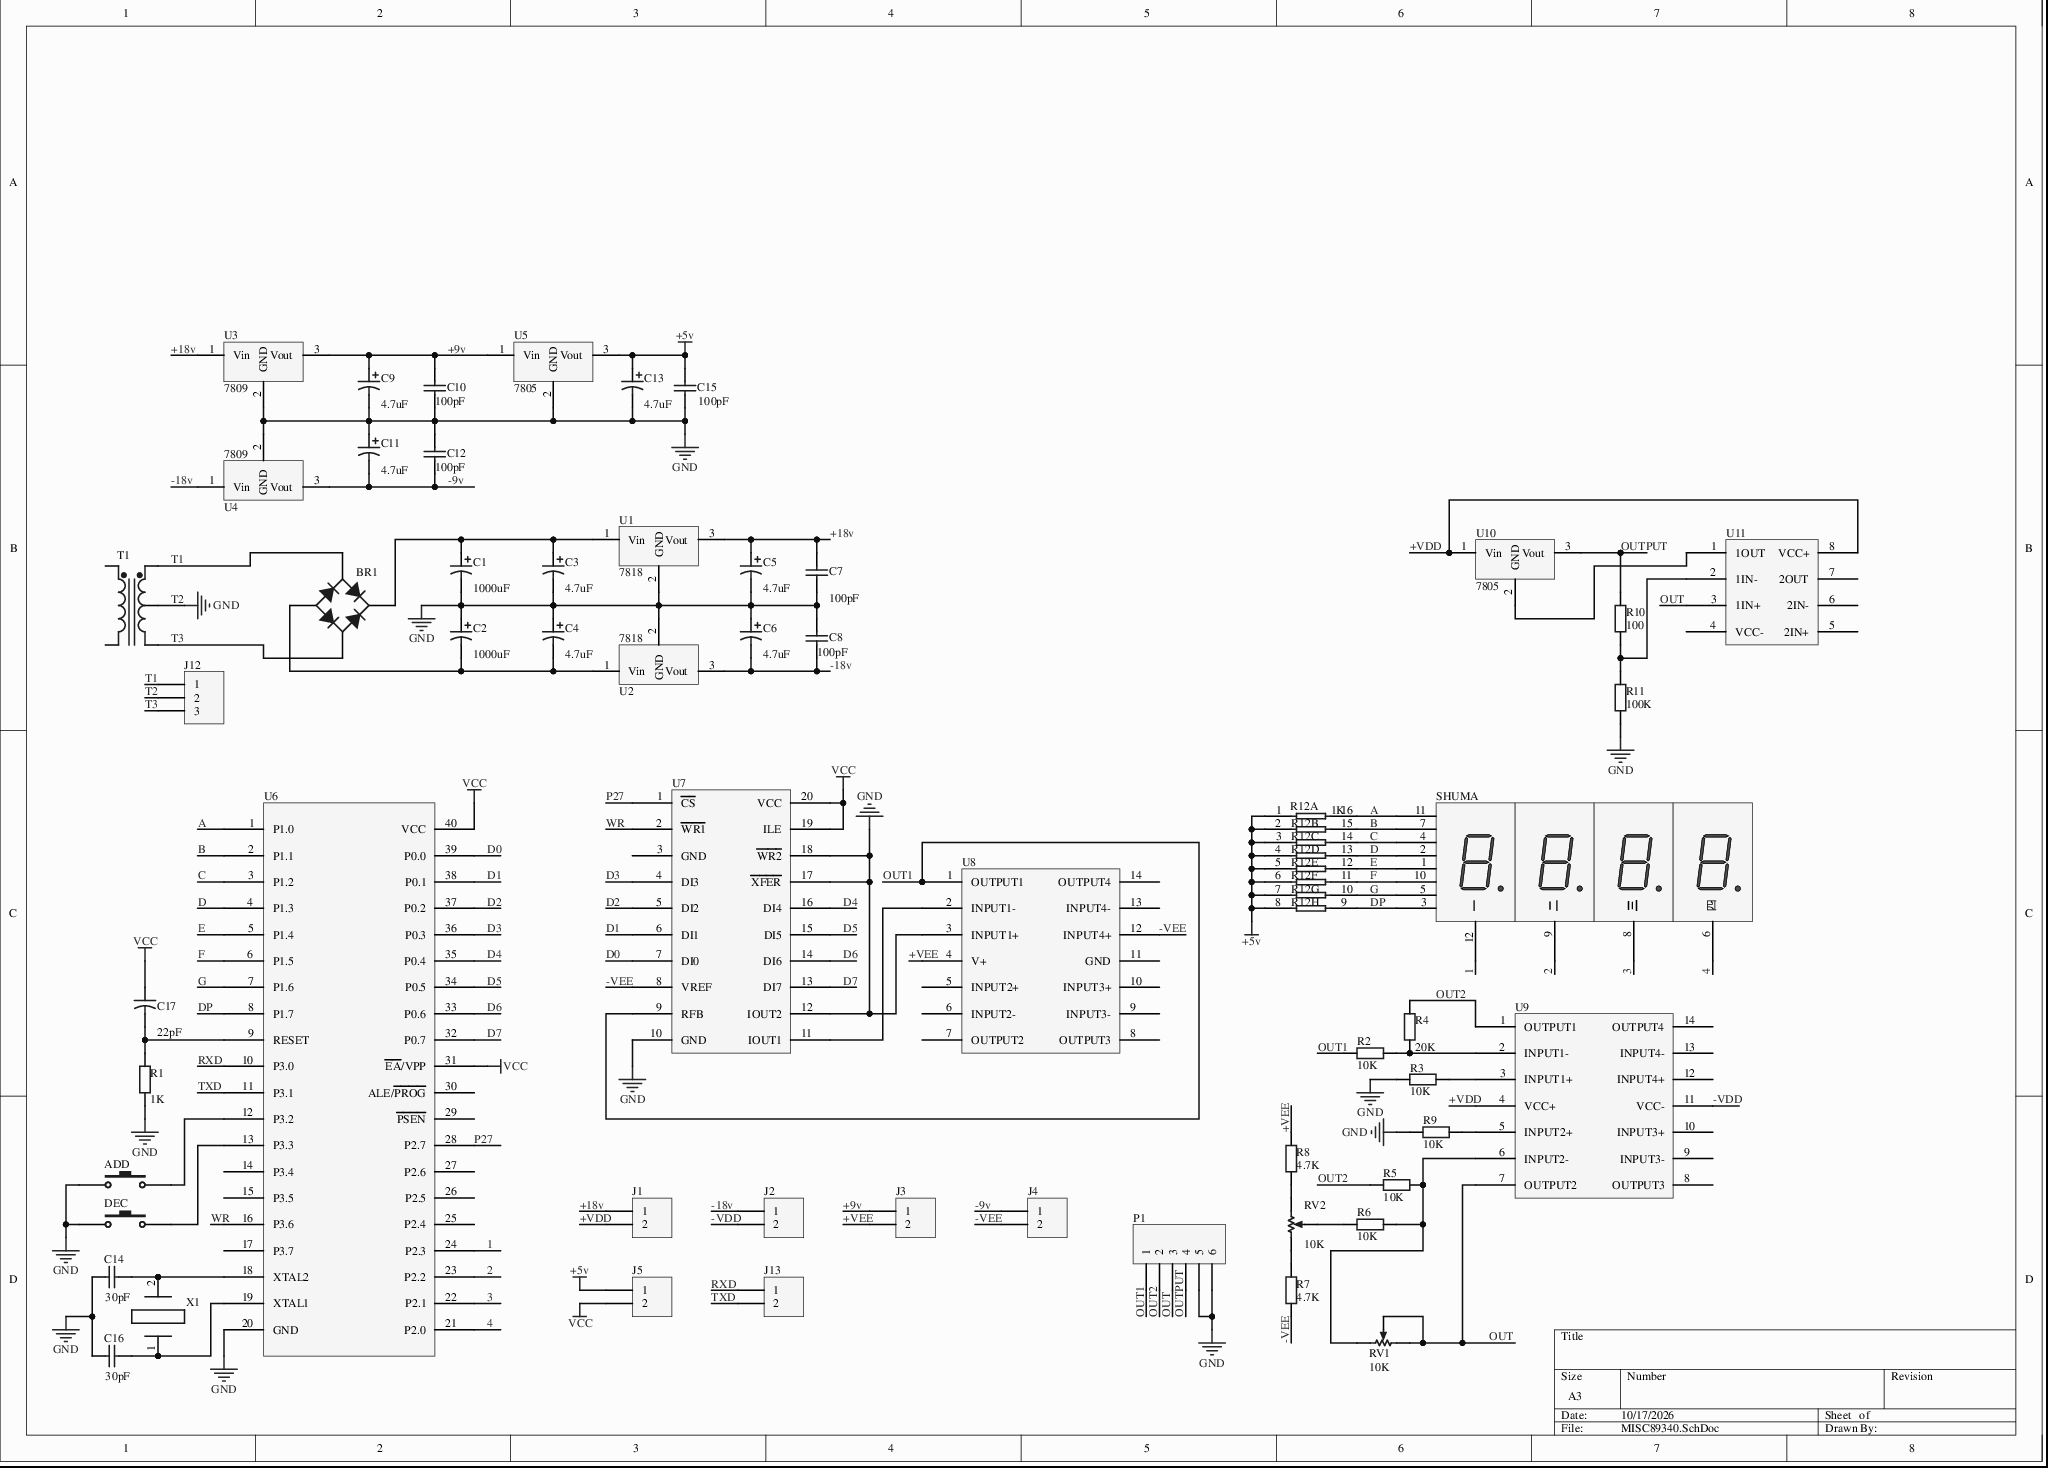
[diagram p0: MISC89340.SchDoc]
# Altium project MISC89340.PrjPcb
1 sheet, 56 parts. Net scope: global (net labels, ports and power ports of the same name join across sheets).
Board file: MISC89340.PcbDoc

## Sheet MISC89340.SchDoc
size A3

### Parts
ADD  SW-PB  [SPST-2]  (value not drawn)
BR1  Bridge1  [LC-KBP]  (value not drawn)
C1  value 1000uF  [RB7.6-15]  (hidden comment: Cap Pol1)
C2  value 1000uF  [RB7.6-15]  (hidden comment: Cap Pol1)
C3  value 4.7uF  [RB7.6-15]  (hidden comment: Cap Pol1)
C4  value 4.7uF  [RB7.6-15]  (hidden comment: Cap Pol1)
C5  value 4.7uF  [RB7.6-15]  (hidden comment: Cap Pol1)
C6  value 4.7uF  [RB7.6-15]  (hidden comment: Cap Pol1)
C7  value 100pF  [RAD-0.3]  (hidden comment: Cap)
C8  value 100pF  [RAD-0.3]  (hidden comment: Cap)
C9  value 4.7uF  [RB7.6-15]  (hidden comment: Cap Pol1)
C10  value 100pF  [RAD-0.3]  (hidden comment: Cap)
C11  value 4.7uF  [RB7.6-15]  (hidden comment: Cap Pol1)
C12  value 100pF  [RAD-0.3]  (hidden comment: Cap)
C13  value 4.7uF  [RB7.6-15]  (hidden comment: Cap Pol1)
C14  value 30pF  [RAD-0.3]  (hidden comment: Cap)
C15  value 100pF  [RAD-0.3]  (hidden comment: Cap)
C16  value 30pF  [RAD-0.3]  (hidden comment: Cap)
C17  value 22pF  [CAPR5-4X5]  (hidden comment: Cap2)
DEC  SW-PB  [SPST-2]  (value not drawn)
J1  Header 2  [HDR1X2]  (value not drawn)
J2  Header 2  [HDR1X2]  (value not drawn)
J3  Header 2  [HDR1X2]  (value not drawn)
J4  Header 2  [HDR1X2]  (value not drawn)
J5  Header 2  [HDR1X2]  (value not drawn)
J12  Header 3  [HDR1X3]  (value not drawn)
J13  Header 2  [HDR1X2]  (value not drawn)
P1  Header 6  [HDR1X6]  (value not drawn)
R1  value 1K  [AXIAL-0.4]  (hidden comment: Res2)
R2  value 10K  [AXIAL-0.4]  (hidden comment: Res2)
R3  value 10K  [AXIAL-0.4]  (hidden comment: Res2)
R4  value 20K  [AXIAL-0.4]  (hidden comment: Res2)
R5  value 10K  [AXIAL-0.4]  (hidden comment: Res2)
R6  value 10K  [AXIAL-0.4]  (hidden comment: Res2)
R7  value 4.7K  [AXIAL-0.4]  (hidden comment: Res2)
R8  value 4.7K  [AXIAL-0.4]  (hidden comment: Res2)
R9  value 10K  [AXIAL-0.4]  (hidden comment: Res2)
R10  value 100  [AXIAL-0.4]  (hidden comment: Res2)
R11  value 100K  [AXIAL-0.4]  (hidden comment: Res2)
R12  value 1K  [DIP-16]  (hidden comment: Res Pack2)  (parts A,B,C,D,E,F,G,H of 8)
RV1  value 10K  [VR5]  (hidden comment: RPot)
RV2  value 10K  [VR5]  (hidden comment: RPot)
SHUMA  Dpy Red-CA  [四位数码管]  (value not drawn)
T1  Trans CT  [TRF_5]  (value not drawn)
U1  7818  [7805]
U2  7818  [7805]
U3  7809  [7805]
U4  7809  [7805]
U5  7805  [7805]
U6  89c51  [89c51]  (value not drawn)
U7  Component_1  [DAC0832]  (value not drawn)
U8  Component_1  [LM324]  (value not drawn)
U9  Component_1  [TL084]  (value not drawn)
U10  7805  [7805]
U11  (no value)  [NE5532]
X1  Component_1  [LC-HC-49S]  (value not drawn)

### Nets
+5v: C13.1 C15.2 J5.1 R12.1 R12.2 R12.3 R12.4 R12.5 R12.6 R12.7 R12.8 U5.3(Vout)
T2: ADD.1 C1.2 C2.1 C3.2 C4.1 C5.2 C6.1 C7.1 C8.2 C9.2 C10.1 C11.1 C12.2 C13.2 C14.1 C15.1 C16.1 DEC.1 J12.2 P1.5 P1.6 R1.1 R3.2 R9.2 R11.2 T1.4(SecCT) U1.2(GND) U2.2(GND) U3.2(GND) U4.2(GND) U5.2(GND) U6.20(GND) U7.10(GND) U7.12(IOUT2) U7.17(~{XFER}) U7.18(~{WR2}) U8.3(INPUT1+)  [also labelled GND]
VCC: C17.1 J5.2 U6.31(~{EA}/VPP) U6.40(VCC) U7.19(ILE) U7.20(VCC)
1: SHUMA.12(一) U6.24(P2.3)
2: SHUMA.9(二) U6.23(P2.2)
3: SHUMA.8(三) U6.22(P2.1)
4: SHUMA.6(四) U6.21(P2.0)
+9v: C9.1 C10.2 J3.1 U3.3(Vout) U5.1(Vin)
+18v: C5.1 C7.2 J1.1 U1.3(Vout) U3.1(Vin)
+VDD: J1.2 U9.4(VCC+) U10.1(Vin) U11.8(VCC+)
+VEE: J3.2 R8.1 U8.4(V+)
-9v: C11.2 C12.1 J4.1 U4.3(Vout)
-18v: C6.2 C8.1 J2.1 U2.3(Vout) U4.1(Vin)
-VDD: J2.2 U9.11(VCC-)
-VEE: J4.2 R7.2 U7.8(VREF) U8.12(INPUT4+)
A: R12.16 SHUMA.11 U6.1(P1.0)
B: R12.15 SHUMA.7 U6.2(P1.1)
C: R12.14 SHUMA.4 U6.3(P1.2)
D: R12.13 SHUMA.2 U6.4(P1.3)
D0: U6.39(P0.0) U7.7(DI0)
D1: U6.38(P0.1) U7.6(DI1)
D2: U6.37(P0.2) U7.5(DI2)
D3: U6.36(P0.3) U7.4(DI3)
D4: U6.35(P0.4) U7.16(DI4)
D5: U6.34(P0.5) U7.15(DI5)
D6: U6.33(P0.6) U7.14(DI6)
D7: U6.32(P0.7) U7.13(DI7)
DP: R12.9 SHUMA.3 U6.8(P1.7)
E: R12.12 SHUMA.1 U6.5(P1.4)
F: R12.11 SHUMA.10 U6.6(P1.5)
G: R12.10 SHUMA.5 U6.7(P1.6)
OUT: P1.3 RV1.1(TOP) RV1.3(TAP) U9.7(OUTPUT2) U11.3(1IN+)
OUT1: P1.1 R2.2 U7.9(RFB) U8.1(OUTPUT1)
OUT2: P1.2 R4.2 R5.2 U9.1(OUTPUT1)
OUTPUT: P1.4 R10.1 U10.3(Vout)
P27: U6.28(P2.7) U7.1(~{CS})
RXD: J13.1 U6.10(P3.0)
T1: BR1.4(C) J12.1 T1.3(Sec+)
T3: BR1.2(C) J12.3 T1.5(Sec-)
TXD: J13.2 U6.11(P3.1)
WR: U6.16(P3.6) U7.2(~{WR1})
NetADD_2: ADD.2 U6.12(P3.2)
NetBR1_1: BR1.1(K) C1.1 C3.1 U1.1(Vin)
NetBR1_3: BR1.3(A) C2.2 C4.2 U2.1(Vin)
NetC14_2: C14.2 U6.18(XTAL2) X1.2
NetC16_2: C16.2 U6.19(XTAL1) X1.1
NetC17_2: C17.2 R1.2 U6.9(RESET)
NetDEC_2: DEC.2 U6.13(P3.3)
NetR2_1: R2.1 R4.1 U9.2(INPUT1-)
NetR3_1: R3.1 U9.3(INPUT1+)
NetR5_1: R5.1 R6.1 RV1.2(BOT) U9.6(INPUT2-)
NetR6_2: R6.2 RV2.3(TAP)
NetR7_1: R7.1 RV2.1(TOP)
NetR8_2: R8.2 RV2.2(BOT)
NetR9_1: R9.1 U9.5(INPUT2+)
NetR10_2: R10.2 R11.1 U11.2(1IN-)
NetU7_11: U7.11(IOUT1) U8.2(INPUT1-)
NetU10_2: U10.2(GND) U11.1(1OUT)

Not connected (* = marked no-connect by the designer): T1 1(Pri+) 2(Pri-); U6 14(P3.4) 15(P3.5) 17(P3.7) 25(P2.4) 26(P2.5) 27(P2.6) 29(~{PSEN}) 30(ALE/~{PROG}); U7 3(GND); U8 5(INPUT2+) 6(INPUT2-) 7(OUTPUT2) 8(OUTPUT3) 9(INPUT3-) 10(INPUT3+) 11(GND) 13(INPUT4-) 14(OUTPUT4); U9 8(OUTPUT3) 9(INPUT3-) 10(INPUT3+) 12(INPUT4+) 13(INPUT4-) 14(OUTPUT4); U11 4(VCC-) 5(2IN+) 6(2IN-) 7(2OUT)

### Library data of the parts
ADD DEC = SW-PB: Switch; Published: 24-Mar-1999; LatestRevisionDate: 17-Jul-2002; LatestRevisionNote: Re-released for DXP Platform.; PackageReference: SPST-2; PackageDescription: Switch; 2 Leads; Publisher: Altium Limited
BR1 = Bridge1: Full Wave Diode Bridge; Published: 8-Jun-2000; LatestRevisionDate: 29-May-2009; LatestRevisionNote: Sch pins A & K swapped.; DatasheetVersion: E2732B; PackageReference: D-38; PackageDescription: Bridge Rectifier; 4 Terminals; Body 9.4 x 9.4 mm (typ); Pitch 5.08 mm; Publisher: Altium Limited
C1-C6 C9 C11 C13 = Cap Pol1: Polarized Capacitor (Radial); Published: 8-Jun-2000; LatestRevisionDate: 17-Jul-2002; LatestRevisionNote: Re-released for DXP Platform.; PackageReference: RB7.6-15; PackageDescription: Polarized Capacitor (Radial); 2 Leads; Publisher: Altium Limited
C7 C8 C10 C12 C14-C16 = Cap: Capacitor; Published: 8-Jun-2000; LatestRevisionDate: 17-Jul-2002; LatestRevisionNote: Re-released for DXP Platform.; PackageReference: RAD-0.3; PackageDescription: Radial Cap, Thru-Hole; 2 Leads; 0.3 in Pin Spacing; Publisher: Altium Limited
C17 = Cap2: Capacitor; Published: 23-Sep-2002; PackageReference: CAPR5-4X5; PackageDescription: Capacitor; 2 Leads; Publisher: Altium Limited
J1-J5 J13 = Header 2: Header, 2-Pin; LatestRevisionDate: 17-Jul-2002; LatestRevisionNote: Re-released for DXP Platform.; Publisher: Altium Limited
J12 = Header 3: Header, 3-Pin; LatestRevisionDate: 17-Jul-2002; LatestRevisionNote: Re-released for DXP Platform.; Publisher: Altium Limited
P1 = Header 6: Header, 6-Pin; LatestRevisionDate: 17-Jul-2002; LatestRevisionNote: Re-released for DXP Platform.; Publisher: Altium Limited
R1-R11 = Res2: Resistor; Published: 8-Jun-2000; LatestRevisionDate: 17-Jul-2002; LatestRevisionNote: Re-released for DXP Platform.; PackageReference: AXIAL-0.4; PackageDescription: Axial Device, Thru-Hole; 2 Leads; 0.4 in Pin Spacing; Publisher: Altium Limited
R12 = Res Pack2: Isolated Resistor Network - Parts; Sim Note: Enter the Resistance value into parameter field.; Published: 24-Mar-1999; LatestRevisionDate: 17-Jul-2002; LatestRevisionNote: Re-released for DXP Platform.; PackageReference: DIP-16; Code_JEDEC: MO-001-AC; Publisher: Altium Limited
RV1 RV2 = RPot: Potentiometer; Sim Note: Enter the Resistance value and the set point into parameter fields.; Set Position: 0.5; Published: 8-Jun-2000; LatestRevisionDate: 17-Jul-2002; LatestRevisionNote: Re-released for DXP Platform.; PackageReference: VR5; PackageDescription: Variable Resistor, Thru-Hole; 3 Leads; Publisher: Altium Limited
SHUMA = Dpy Red-CA: 7.62 mm Black Surface HER 7-Segment Display: CA, RH DP; MinimumIntensity: 360 ucd; Note: IF = 5 mA; Note: Pins 1 and 6 are redundant Anodes.; Published: 8-Jun-2000; LatestRevisionDate: 17-Dec-2003; LatestRevisionNote: Schematic revised, PCB Footprint replaced.; DatasheetVersion: 19-Feb-2002; PackageVersion: 11-Feb-2002; PackageReference: A; PackageDescription: LED, 7-Segment Display, 7.62 mm, RHD; 10 Leads; Row Space 5.08 mm; Pitch 2.54 mm; Colour: High Efficiency Red (HER); ComponentLink1Description: Manufacturer Link; Publisher: Altium Limited
T1 = Trans CT: Center-Tapped Transformer (Coupled Inductor Model); Published: 8-Jun-2000; LatestRevisionDate: 17-Jul-2002; LatestRevisionNote: Re-released for DXP Platform.; PackageReference: TRF_5; PackageDescription: Transformer; 5 Leads; Publisher: Altium Limited
U1-U5 U10 = Volt Reg: Voltage Regulator; Published: 24-Mar-1999; LatestRevisionDate: 29-May-2009; LatestRevisionNote: IPC-7351 Footprint Added.; PackageReference: D2PAK; PackageDescription: 3-Pin Transistor Outline Package 2.54 mm Pitch, 15.1 mm Lead Span; Publisher: Altium Limited
U6 U11 = Component_1